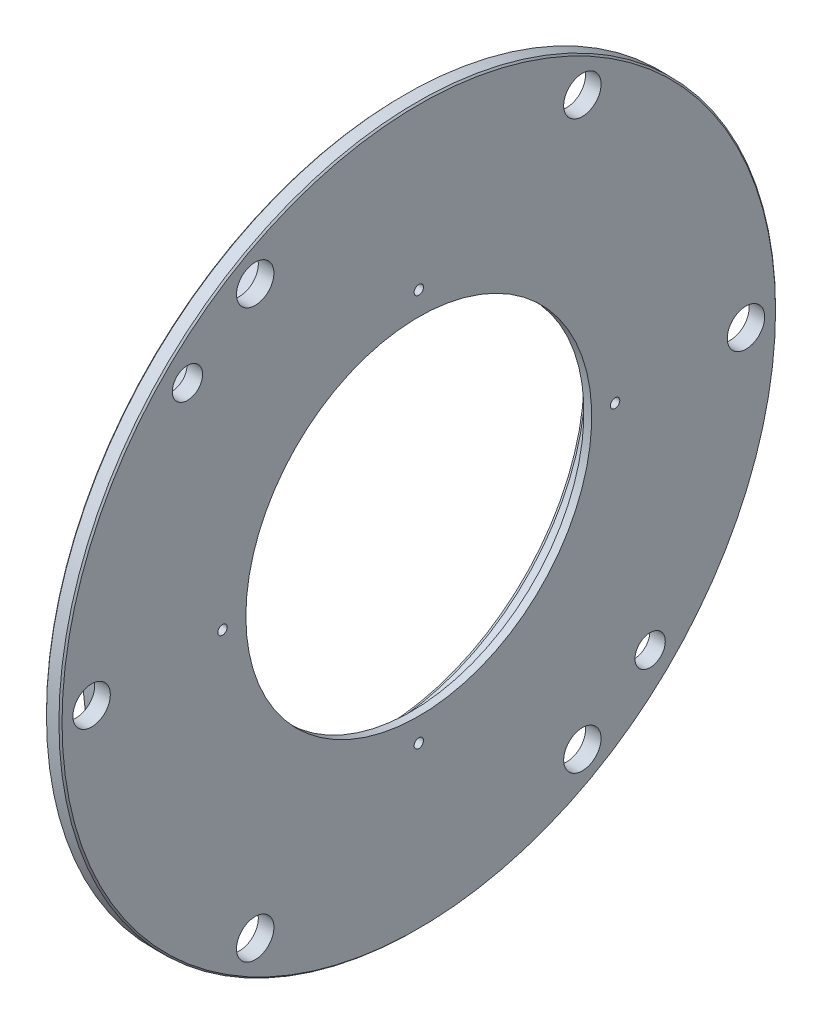
from build123d import *

# Parameters (mm, degrees)
SKETCH3_R              = 12
CUT_EXTRUDE1_DEPTH     = 327.387806145
CIRPATTERN1_COUNT      = 6
SKETCH4_R              = 3
CUT_EXTRUDE5_DEPTH     = 327.387806145
CIRPATTERN2_COUNT      = 4
SKETCH5_R              = 130
CUT_EXTRUDE6_DEPTH     = 22
SKETCH6_R              = 175
CUT_EXTRUDE7_DEPTH     = 2
CHAMFER2_SIZE          = 2
CHAMFER2_SIZE2         = 1.154700538
CHAMFER3_SIZE          = 1
F_7_8_9_TAPPED_HOLE1_D = 19.44624
CIRPATTERN4_COUNT      = 2


with BuildPart() as part:
    # Sketch1 → Revolve1 (revolve)
    with BuildSketch(Plane.XY, mode=Mode.PRIVATE) as revolve1_sk:
        Polygon((0, 111), (0, 230), (-10, 230), (-10, 190), (-27, 190), (-27, 111), align=None)
    revolve(revolve1_sk.sketch.rotate(Axis((-73.563127278, 0, 0), (1, 0, 0)), 90), axis=Axis((-73.563127278, 0, 0), (1, 0, 0)))

    # Sketch3 → Cut-Extrude1 (cut, through all)
    with BuildSketch(Plane(origin=(0, 0, 0), x_dir=(0, 0, -1), z_dir=(1, 0, 0))):
        with Locations((-210, 0)):
            Circle(SKETCH3_R)
    cut_extrude1 = extrude(amount=-CUT_EXTRUDE1_DEPTH, mode=Mode.SUBTRACT)

    # CirPattern1: Cut-Extrude1 ×6 about axis
    cirpattern1_axis = Axis((0, 0, 0), (1, 0, 0))
    for i in range(1, CIRPATTERN1_COUNT):
        add(cut_extrude1.rotate(cirpattern1_axis, i * 360 / CIRPATTERN1_COUNT), mode=Mode.SUBTRACT)

    # Sketch4 → Cut-Extrude5 (cut, through all)
    with BuildSketch(Plane(origin=(0, 0, 0), x_dir=(0, 0, -1), z_dir=(1, 0, 0))):
        with Locations((-126, 0)):
            Circle(SKETCH4_R)
    cut_extrude5 = extrude(amount=-CUT_EXTRUDE5_DEPTH, mode=Mode.SUBTRACT)

    # CirPattern2: Cut-Extrude5 ×4 about axis
    cirpattern2_axis = Axis((0, 0, 0), (1, 0, 0))
    for i in range(1, CIRPATTERN2_COUNT):
        add(cut_extrude5.rotate(cirpattern2_axis, i * 360 / CIRPATTERN2_COUNT), mode=Mode.SUBTRACT)

    # Sketch5 → Cut-Extrude6 (cut)
    with BuildSketch(Plane.ZY.offset(27)):
        Circle(SKETCH5_R)
    extrude(amount=-CUT_EXTRUDE6_DEPTH, mode=Mode.SUBTRACT)

    # Sketch6 → Cut-Extrude7 (cut)
    with BuildSketch(Plane.ZY.offset(27)):
        Circle(SKETCH6_R)
    extrude(amount=-CUT_EXTRUDE7_DEPTH, mode=Mode.SUBTRACT)

    # Chamfer2
    chamfer2_edges = [part.edges().sort_by_distance(p)[0] for p in [
        (-25, 0, -130),
    ]]
    chamfer2_side = [part.faces().sort_by_distance(p)[0] for p in [
        (-15, 0, -130),
    ]]
    chamfer(chamfer2_edges, length=CHAMFER2_SIZE, length2=CHAMFER2_SIZE2, reference=chamfer2_side[0])

    # Chamfer3
    chamfer3_edges = [part.edges().sort_by_distance(p)[0] for p in [
        (0, 0, -230),
        (-27, 0, -190),
        (-10, 0, -230),
    ]]
    chamfer(chamfer3_edges, length=CHAMFER3_SIZE)

    # 7/8-9 Tapped Hole1 (through all)
    with Locations(Plane(origin=(0, 148.492424572, 148.492423527), x_dir=(0, 0, 1), z_dir=(1, 0, 0))):
        with Locations((0, 0)):
            f_7_8_9_tapped_hole1 = Hole(F_7_8_9_TAPPED_HOLE1_D / 2)

    # CirPattern4: 7/8-9 Tapped Hole1 ×2 about axis
    cirpattern4_axis = Axis((0, 0, 0), (1, 0, 0))
    for i in range(1, CIRPATTERN4_COUNT):
        add(f_7_8_9_tapped_hole1.rotate(cirpattern4_axis, i * 360 / CIRPATTERN4_COUNT), mode=Mode.SUBTRACT)


solid = part.part
